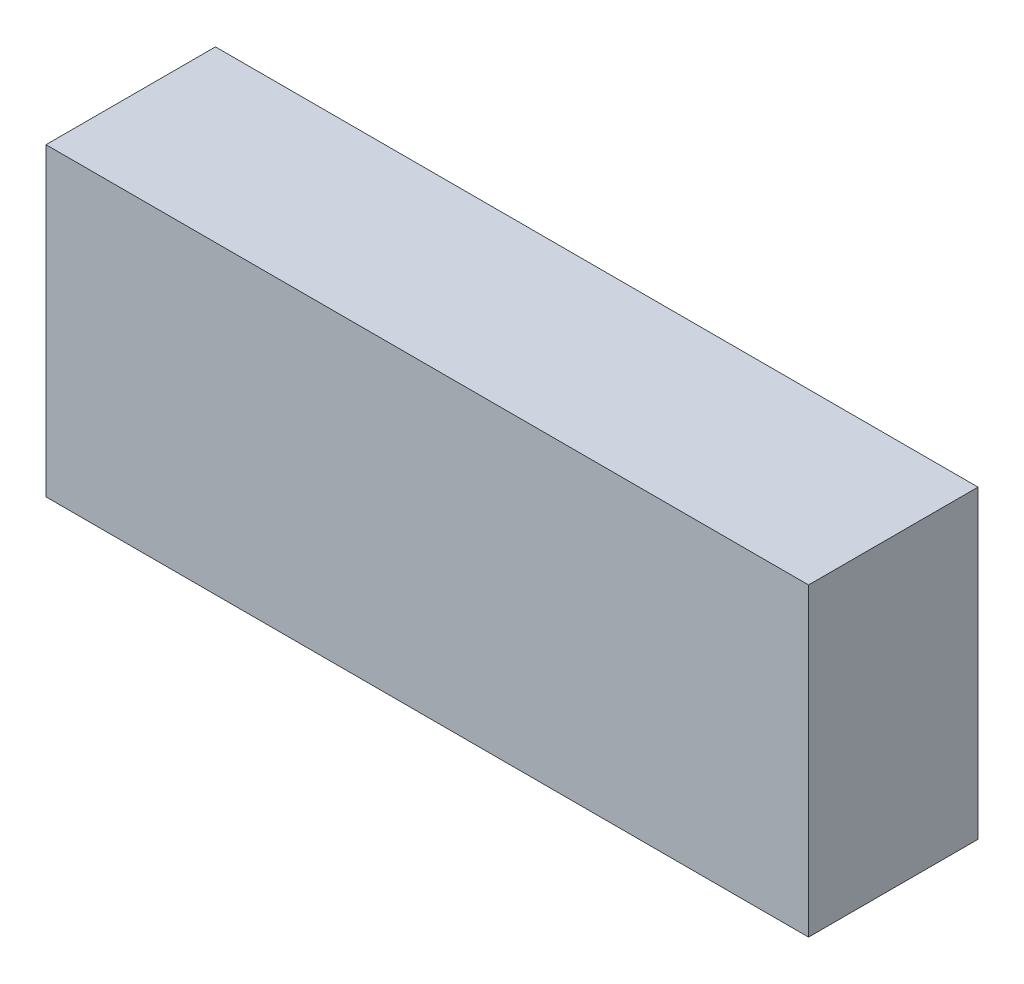
SolidWorks part; units mm, degrees
ref_plane "前视基准面" through (0, 0, 0) normal (0, 0, 1) x (1, 0, 0)
ref_plane "上视基准面" through (0, 0, 0) normal (0, 1, 0) x (1, 0, 0)
ref_plane "右视基准面" through (0, 0, 0) normal (1, 0, 0) x (0, 0, -1)
other "Configuration Table"
sketch "草图1" plane through (0, 0, 0) normal (0, 0, 1) x (1, 0, 0)
  line L0 (-22.5, -9) -> (22.5, -9)
  line L1 (22.5, -9) -> (22.5, 9)
  line L2 (22.5, 9) -> (-22.5, 9)
  line L3 (-22.5, 9) -> (-22.5, -9)
  point P0 (0, 0)
  dimension "D1" = 22.5
  dimension "D2" = 45
  dimension "D3" = 9
  dimension "D4" = 18
extrude "凸台-拉伸1" add sketch "草图1" against normal mid plane 10
